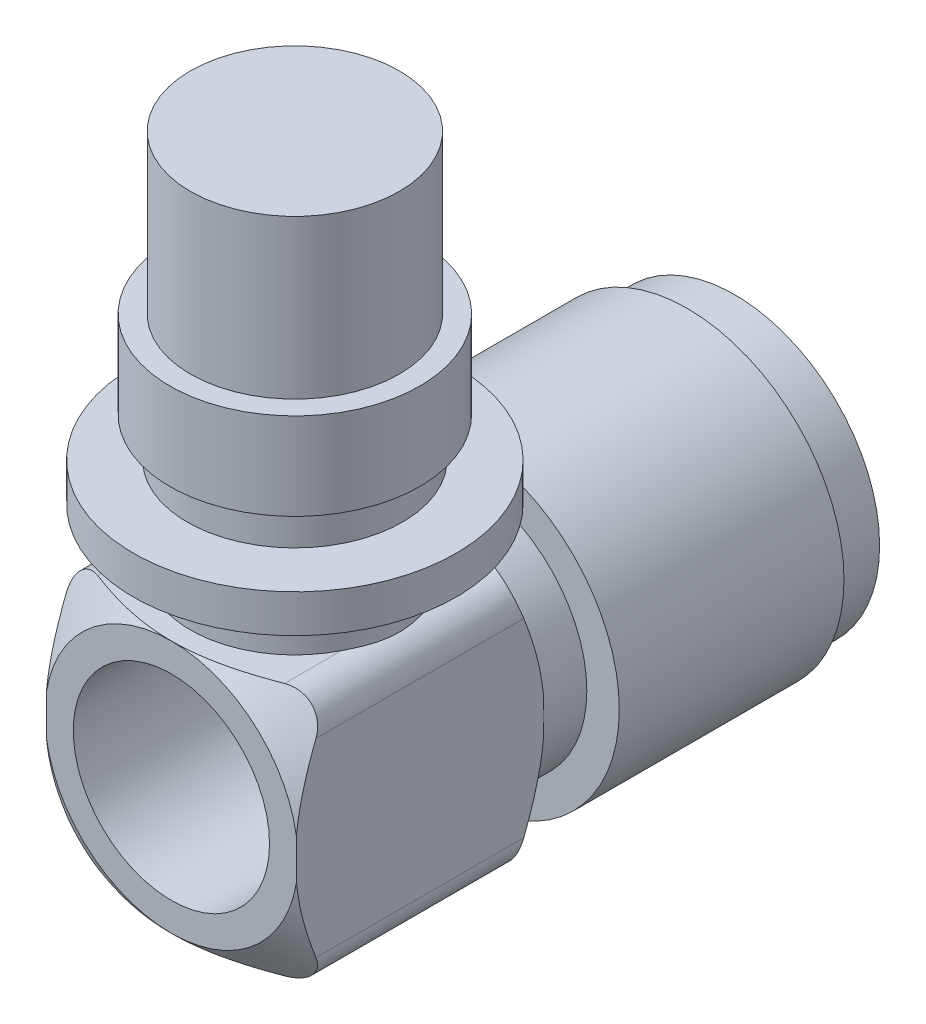
SolidWorks part; units mm, degrees
material "铜"
ref_plane "Front Plane" through (0, 0, 0) normal (0, 0, 1) x (1, 0, 0)
ref_plane "Top Plane" through (0, 0, 0) normal (0, 1, 0) x (1, 0, 0)
ref_plane "Right Plane" through (0, 0, 0) normal (1, 0, 0) x (0, 0, -1)
sketch "Sketch1" plane through (0, 0, 0) normal (0, 1, 0) x (1, 0, 0)
  line L1 (-3.95, -3.9) -> (3.95, -3.9)
  line L2 (-3.95, -3.9) -> (-3.95, 3.9)
  line L3 (-3.95, 3.9) -> (3.95, 3.9)
  line L4 (3.95, -3.9) -> (3.95, 3.9)
  line L5 (-3.95, -3.9) -> (3.95, 3.9) construction
  line L6 (-3.95, 3.9) -> (3.95, -3.9) construction
  point P0 (0, 0)
  dimension "D1" = 7.9
  dimension "D2" = 7.8
extrude "Boss-Extrude1" add sketch "Sketch1" along normal blind 8
fillet "Fillet1" radius 1 4 edges at (-3.95, 0, 0) (3.95, 0, 0) (-3.95, 8, 0) (3.95, 8, 0)
sketch "Sketch2" plane through (0, 0, 0) normal (1, 0, 0) x (0, 0, -1)
  line L0 (-3.9, 4) -> (5.3985, 4) construction
  line L6 (-3.9, 7) -> (-3.9, 1) construction
ref_plane "Plane1" through (-2, 2, 0) normal (0.7071, -0.7071, 0) x (0, 0, -1)
sketch "Sketch3" plane through (-2, 2, 0) normal (0.7071, -0.7071, 0) x (0, 0, -1)
  line L0 (3, 8.2284) -> (4, 8.2284)
  line L2 (4, 8.2284) -> (3.9, 6.8284)
  line L3 (3.9, 7.7428) -> (3.9, 3.5002) construction
  line L4 (3.9, 6.8284) -> (3, 8.2284)
  line L5 (-3.9, 2.8284) -> (5.3985, 2.8284) construction
  line L6 (3.9, 7.7428) -> (-3.9, 7.7428) construction
  dimension "D1" = 1
  dimension "D3" = 4
  dimension "D4" = 0.4856
revolve "Cut-Revolve4" cut sketch "Sketch3" angle 360 about L0
mirror "Mirror2" about plane through (0, 0, 0) normal (0, 0, 1) of "Cut-Revolve4"
ref_plane "Plane2" through (0, 20, 0) normal (0, 1, 0) x (1, 0, 0)
sketch "Sketch4" plane through (0, 20, 0) normal (0, 1, 0) x (1, 0, 0)
  circle A0 centre (0, 0) radius 3.3
  dimension "D1" = 6.6
extrude "Boss-Extrude2" add sketch "Sketch4" against normal up to next
sketch "Sketch5" plane through (0, 0, 0) normal (1, 0, 0) x (0, 0, -1)
  line L0 (0, -3.247) -> (0, 22.6942) construction
  line L1 (-5.1, 11) -> (-5.1, 9.8)
  line L2 (-5.1, 11) -> (-3.4, 11)
  line L3 (-5.1, 9.8) -> (-3.3, 9.8)
  line L4 (-3.3, 15) -> (-3.3, 9.8)
  line L5 (-3.3, 20) -> (-3.3, 8) construction
  line L7 (-3.95, 12.25) -> (-3.95, 15)
  line L8 (-3.95, 15) -> (-3.3, 15)
  line L9 (-3.95, 12.25) -> (-3.4, 12.25)
  line L10 (-3.4, 12.25) -> (-3.4, 11)
  line L11 (3.2763, 0) -> (-3.2763, 0) construction
  dimension "D1" = 11
  dimension "D2" = 10.2
  dimension "D3" = 1.2
  dimension "D4" = 4
  dimension "D5" = 7.9
  dimension "D6" = 1.25
  dimension "D7" = 6.8
revolve "Revolve1" add sketch "Sketch5" angle 360 about L0
sketch "Sketch6" plane through (0, 0, -3.9) normal (0, 0, -1) x (-1, 0, 0)
  circle A0 centre (0, 4) radius 3.925
  dimension "D1" = 7.85
extrude "Boss-Extrude3" add sketch "Sketch6" along normal blind 6.75
sketch "Sketch8" plane through (0, 0, 0) normal (1, 0, 0) x (0, 0, -1)
  line L0 (-5.444, 4) -> (16.1736, 4) construction
  line L1 (5.3, 4) -> (5.3, 8.95)
  line L3 (5.3, 8.95) -> (12.4, 8.95)
  line L4 (13.9, 8.575) -> (13.9, 7.6875)
  line L5 (13.2, 4) -> (5.3, 4)
  line L6 (3.9, 0.075) -> (3.9, 7.925) construction
  line L7 (12.4, 8.95) -> (12.4, 8.575)
  line L8 (12.4, 8.575) -> (13.9, 8.575)
  line L9 (12.8876, 6.8) -> (10.65, 6.8)
  line L10 (10.65, 0.075) -> (10.65, 7.925) construction
  line L11 (10.65, 6.8) -> (10.65, 4.4703)
  line L12 (10.65, 4.4703) -> (12.3854, 4.4703)
  line L13 (12.3854, 4.4703) -> (13.2, 4)
  line L14 (13.9, 7.6875) -> (13.4, 7.6875)
  line L15 (13.4, 7.6875) -> (12.8876, 6.8)
  dimension "D1" = 9.9
  dimension "D2" = 1.4
  dimension "D3" = 9.15
  dimension "D4" = 1.5
  dimension "D5" = 30
  dimension "D7" = 8.6
  dimension "D8" = 5.6
  dimension "D9" = 120
  dimension "D10" = 0.5
revolve "Revolve2" add sketch "Sketch8" angle 360 about L0
sketch "Sketch9" plane through (0, 0, 3.9) normal (0, 0, 1) x (1, 0, 0)
  circle A0 centre (0, 4) radius 3.1
  dimension "D1" = 6.2
extrude "Cut-Extrude1" cut sketch "Sketch9" against normal blind 5
